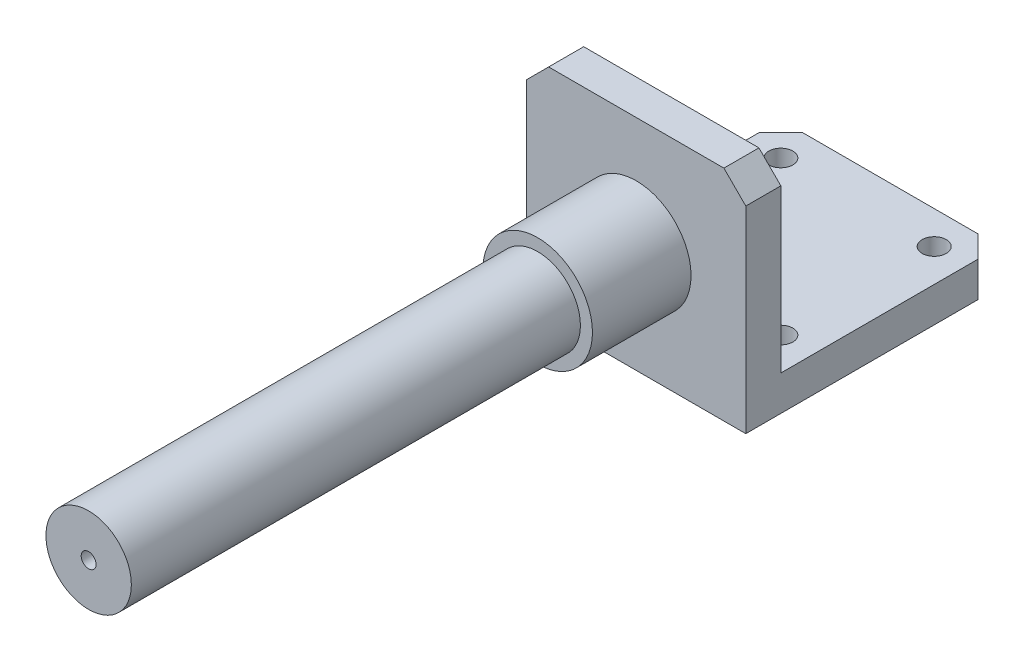
from build123d import *

# Parameters (mm, degrees)
SKETCH_1_W             = 100
SKETCH_1_H             = 100
EXTRUDE_1_DEPTH        = 16
SKETCH_2_R             = 25
EXTRUDE_2_DEPTH        = 250
SKETCH_3_OUTSIDE_W     = 162.252
SKETCH_3_OUTSIDE_H     = 162.252
SKETCH_3_OUTSIDE_R     = 19.5
CUT_EXTRUDE_1_DEPTH    = 205
SKETCH_8_W             = 100
SKETCH_8_H             = 16
EXTRUDE_3_DEPTH        = 100
HOLE_WIZARD_M8_1_D     = 6.8
HOLE_WIZARD_M8_1_DEPTH = 19.75
HOLE_WIZARD_M8_1_TIP   = 2.042926105
HOLE_WIZARD_M10_1_D    = 11
CHAMFER_1_SIZE         = 10


with BuildPart() as part:
    # 草图1 → 凸台-拉伸1 (new body)
    with BuildSketch(Plane.XY):
        Rectangle(SKETCH_1_W, SKETCH_1_H)
    extrude(amount=EXTRUDE_1_DEPTH)

    # 草图2 → 凸台-拉伸2 (add)
    with BuildSketch(Plane.XY.offset(16)):
        Circle(SKETCH_2_R)
    extrude(amount=EXTRUDE_2_DEPTH)

    # 草图3 outside → 切除-拉伸1 (cut)
    with BuildSketch(Plane.XY.offset(266)):
        Rectangle(SKETCH_3_OUTSIDE_W, SKETCH_3_OUTSIDE_H)
        Circle(SKETCH_3_OUTSIDE_R, mode=Mode.SUBTRACT)
    extrude(amount=-CUT_EXTRUDE_1_DEPTH, mode=Mode.SUBTRACT)

    # 草图8 → 凸台-拉伸3 (add)
    with BuildSketch(Plane(origin=(0, 0, 0), x_dir=(-1, 0, 0), z_dir=(0, 0, -1))):
        with Locations((0, -42)):
            Rectangle(SKETCH_8_W, SKETCH_8_H)
    extrude(amount=EXTRUDE_3_DEPTH)

    # M8 螺纹孔1
    with Locations(Plane.XY.offset(266)):
        with Locations((0, 0)):
            Hole(HOLE_WIZARD_M8_1_D / 2, depth=HOLE_WIZARD_M8_1_DEPTH)
            with Locations((0, 0, -(HOLE_WIZARD_M8_1_DEPTH + HOLE_WIZARD_M8_1_TIP / 2))):  # 118° drill point
                Cone(0, HOLE_WIZARD_M8_1_D / 2, HOLE_WIZARD_M8_1_TIP, mode=Mode.SUBTRACT)

    # M10 间隙孔1 (through all)
    with Locations(Plane(origin=(0, -34, -18), x_dir=(1, 0, 0), z_dir=(0, 1, 0))):
        with Locations((-35, 67), (35, 67), (35, -3), (-35, -3)):
            Hole(HOLE_WIZARD_M10_1_D / 2)

    # 倒角1
    chamfer_1_edges = [part.edges().sort_by_distance(p)[0] for p in [
        (-50, -42, -100),
        (50, -42, -100),
        (-50, 50, 8),
        (50, 50, 8),
    ]]
    chamfer(chamfer_1_edges, length=CHAMFER_1_SIZE)


solid = part.part
